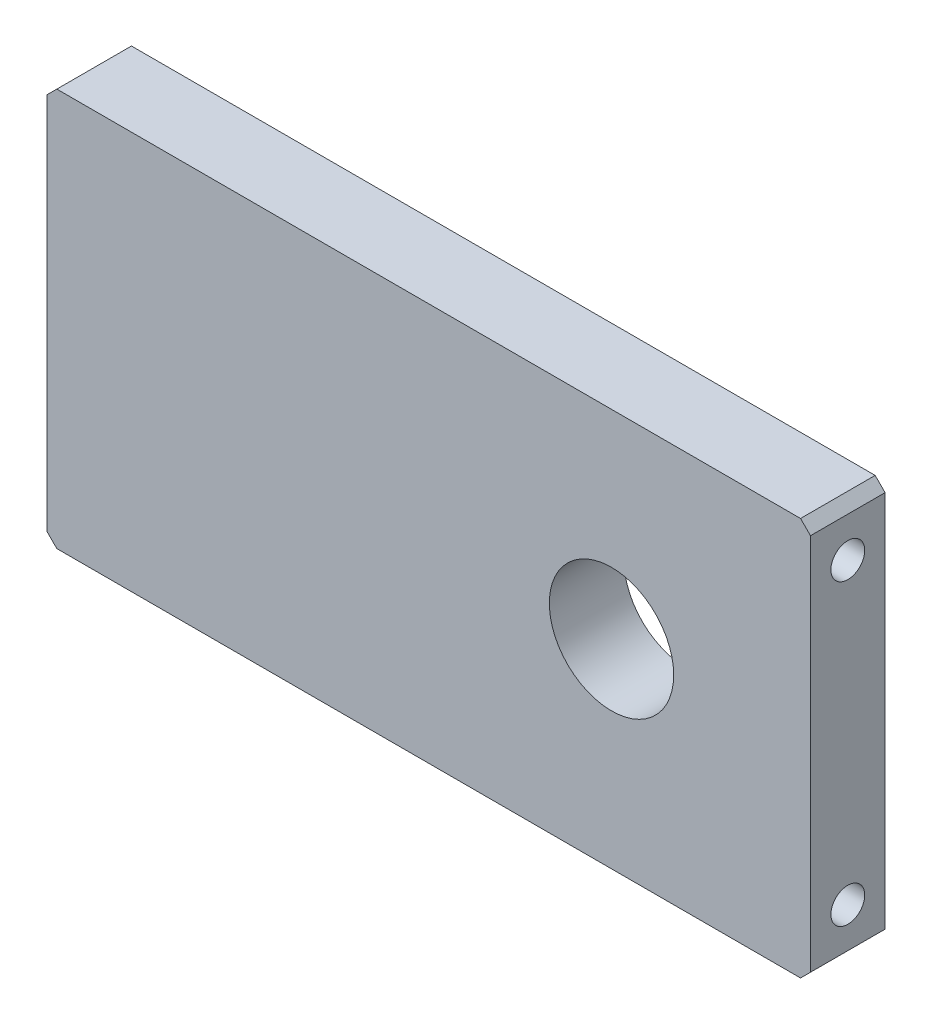
from build123d import *

# Parameters (mm, degrees)
SKETCH_1_W                  = 153.5
SKETCH_1_H                  = 80
EXTRUDE_1_DEPTH             = 7.5
HOLE_WIZARD_25_0_25_1_D     = 25
HOLE_WIZARD_M8_1_AT_2_COUNT = 2
HOLE_WIZARD_M8_1_AT_2_PITCH = 60
SKETCH_6_R                  = 56
CUT_EXTRUDE_1_DEPTH         = 10
CHAMFER_1_SIZE              = 2


with BuildPart() as part:
    # 草图1 → 凸台-拉伸1 (new, symmetric)
    with BuildSketch(Plane.XY):
        Rectangle(SKETCH_1_W, SKETCH_1_H)
    extrude(amount=EXTRUDE_1_DEPTH, both=True)

    # Ø25.0 (25) 直径孔1 (through all)
    with Locations(Plane.XY.offset(7.5)):
        with Locations((36.75, 0)):
            Hole(HOLE_WIZARD_25_0_25_1_D / 2)

    # 草图4 → M8 螺纹孔1 (revolve, cut)
    with BuildSketch(Plane(origin=(76.75, -30, 0), x_dir=(0, 0, -1), z_dir=(0, 1, 0))):
        Polygon((0, 0), (0, 21.792926105), (3.4, 19.75), (3.4, 0), align=None)
    hole_wizard_m8_1 = revolve(axis=Axis((83.1, -30, 0), (-1, 0, 0)), mode=Mode.SUBTRACT)

    # M8 螺纹孔1 at 2: M8 螺纹孔1 ×2
    with Locations(*[(0, i * HOLE_WIZARD_M8_1_AT_2_PITCH, 0) for i in range(1, HOLE_WIZARD_M8_1_AT_2_COUNT)]):
        add(hole_wizard_m8_1, mode=Mode.SUBTRACT)

    # 镜向1: M8 螺纹孔1 across plane
    add(hole_wizard_m8_1.mirror(Plane(origin=(0, 0, 0), x_dir=(0, 0, 1), z_dir=(1, 0, 0))), mode=Mode.SUBTRACT)

    # 镜向1 copy 1 sketch → 镜向1 copy 1 (revolve, cut)
    with BuildSketch(Plane(origin=(-76.75, 30, 0), x_dir=(0, 0, -1), z_dir=(0, 1, 0))):
        Polygon((0, 0), (0, -21.792926105), (3.4, -19.75), (3.4, 0), align=None)
    revolve(axis=Axis((-83.1, 30, 0), (-1, 0, 0)), mode=Mode.SUBTRACT)

    # 草图6 → 切除-拉伸1 (cut)
    with BuildSketch(Plane.ZY.offset(76.75)):
        with Locations((-52.5, 0)):
            Circle(SKETCH_6_R)
    extrude(amount=-CUT_EXTRUDE_1_DEPTH, mode=Mode.SUBTRACT)

    # 倒角1
    chamfer_1_edges = [part.edges().sort_by_distance(p)[0] for p in [
        (76.75, -40, 0),
        (-76.75, -40, 0),
        (-76.75, 40, 0),
        (76.75, 40, 0),
    ]]
    chamfer(chamfer_1_edges, length=CHAMFER_1_SIZE)


solid = part.part
